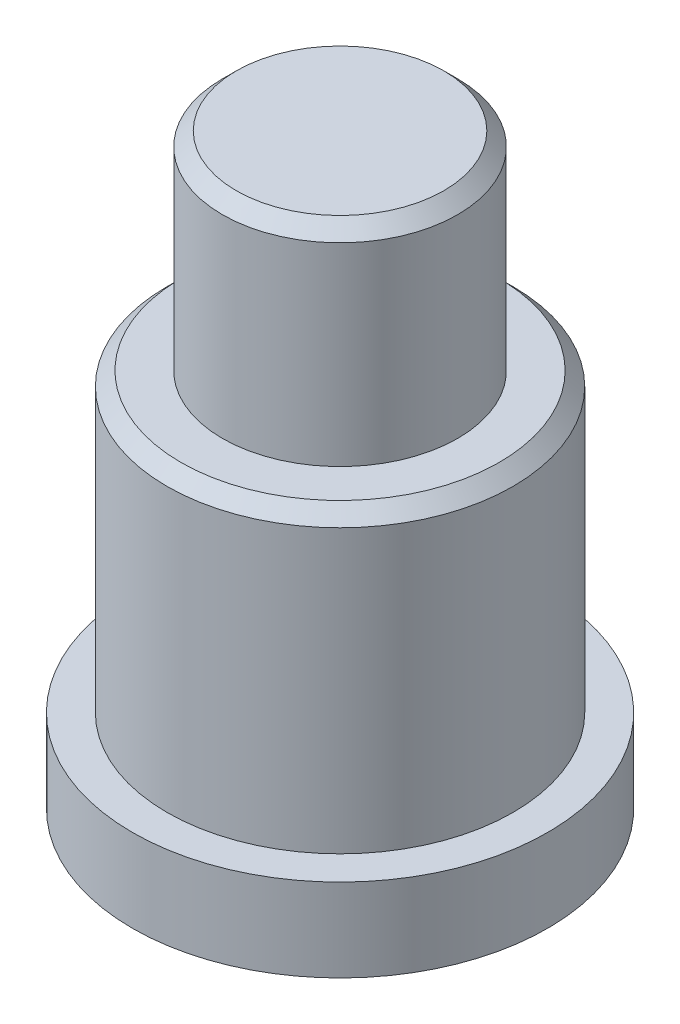
from build123d import *

# Parameters (mm, degrees)
CHAMFER1_SIZE = 0.5


with BuildPart() as part:
    # Sketch1 → Revolve1 (revolve)
    with BuildSketch(Plane.XY, mode=Mode.PRIVATE) as revolve1_sk:
        Polygon((-99.067365632, -10.161784701), (-100.317365632, -10.161784701), (-100.317365632, -13.161784701), (-92.817365632, -13.161784701), (-92.817365632, 8.038215299), (-97.067365632, 8.038215299), (-97.067365632, 0.538215299), (-99.067365632, 0.538215299), align=None)
    revolve(revolve1_sk.sketch.rotate(Axis((-92.817365632, 8.102615299, 0), (0, -1, 0)), 270), axis=Axis((-92.817365632, 8.102615299, 0), (0, -1, 0)))

    # Chamfer1
    chamfer1_edges = [part.edges().sort_by_distance(p)[0] for p in [
        (-92.817365632, 0.538215299, -6.25),
        (-92.817365632, 8.038215299, -4.25),
    ]]
    chamfer(chamfer1_edges, length=CHAMFER1_SIZE)


solid = part.part
